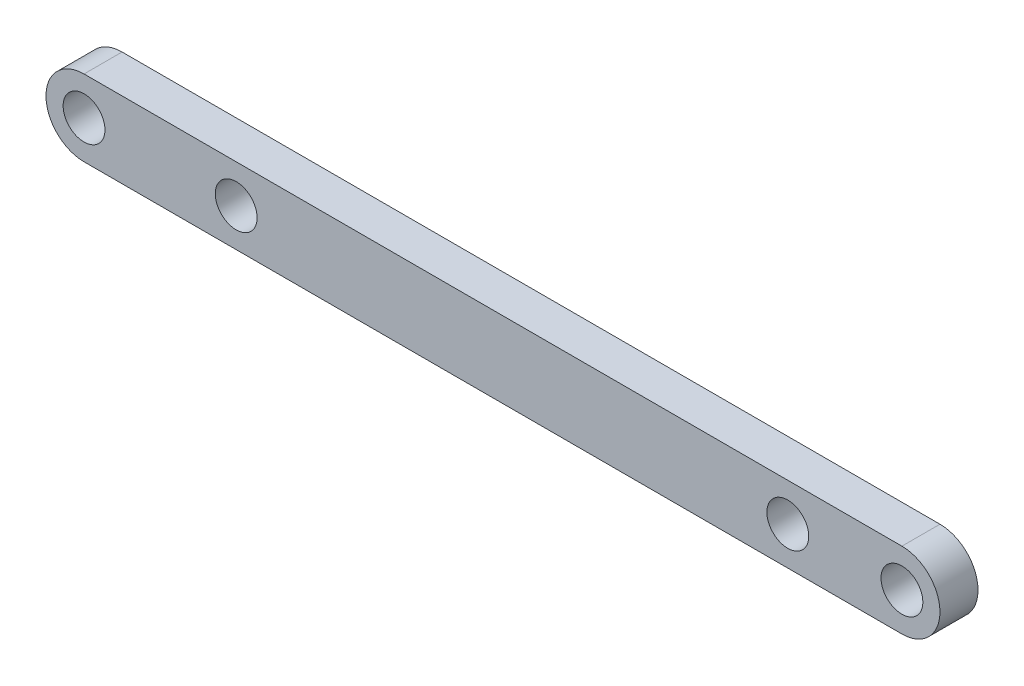
from build123d import *

# Parameters (mm, degrees)
SKETCH1_R           = 0.55
THIGH1_LENGTH_DEPTH = 0.5


with BuildPart() as part:
    # Sketch1 → Thigh1 length (new, symmetric)
    with BuildSketch(Plane.XY):
        with BuildLine():
            Line((-10.75, 1), (10.75, 1))
            ThreePointArc((10.75, 1), (11.75, 0), (10.75, -1))
            Line((10.75, -1), (-10.75, -1))
            ThreePointArc((-10.75, -1), (-11.75, 0), (-10.75, 1))
        make_face()
        with Locations((-10.75, 0)):
            Circle(SKETCH1_R, mode=Mode.SUBTRACT)
        with Locations((10.75, 0)):
            Circle(SKETCH1_R, mode=Mode.SUBTRACT)
        with Locations((-6.75, 0)):
            Circle(SKETCH1_R, mode=Mode.SUBTRACT)
        with Locations((7.75, 0)):
            Circle(SKETCH1_R, mode=Mode.SUBTRACT)
    extrude(amount=THIGH1_LENGTH_DEPTH, both=True)


solid = part.part
